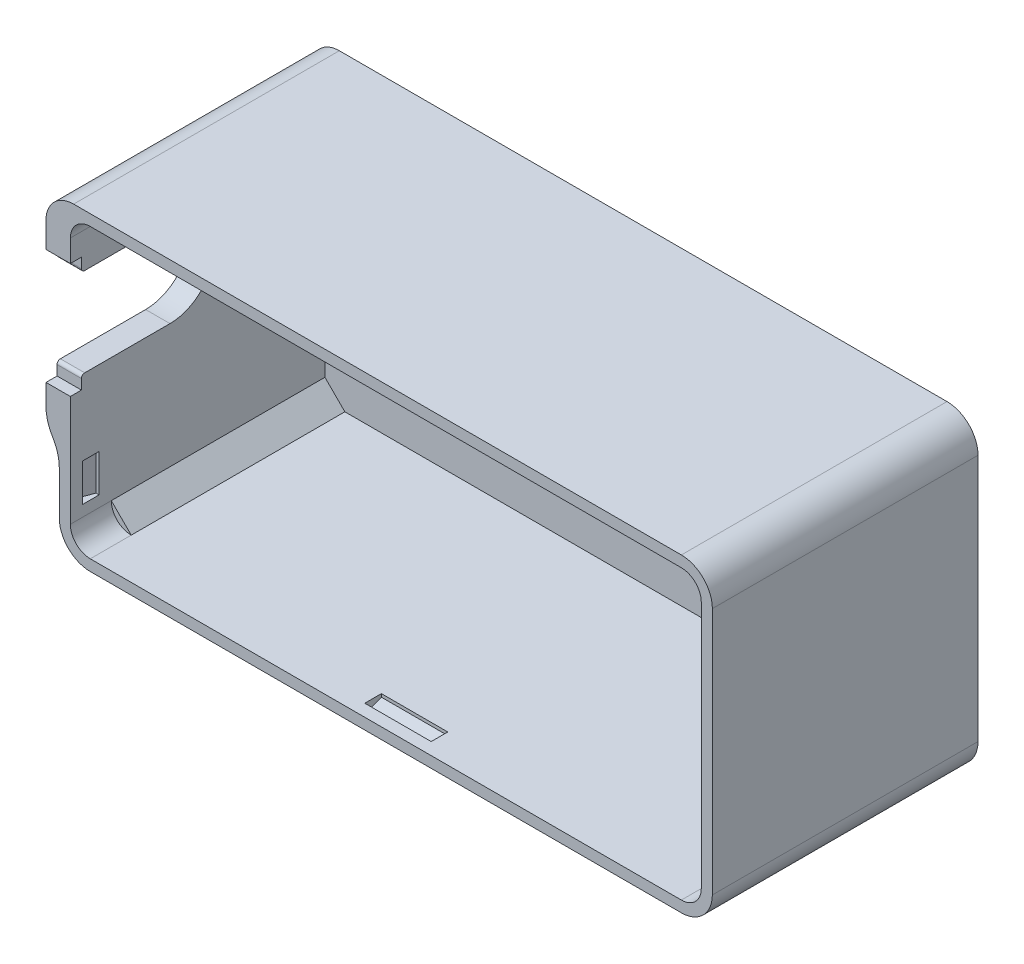
SolidWorks part; units mm, degrees
ref_plane "前视基准面" through (0, 0, 0) normal (0, 0, 1) x (1, 0, 0)
ref_plane "上视基准面" through (0, 0, 0) normal (0, 1, 0) x (1, 0, 0)
ref_plane "右视基准面" through (0, 0, 0) normal (1, 0, 0) x (0, 0, -1)
other "Configuration Table"
sketch "草图1" plane through (0, 0, 0) normal (0, 0, 1) x (1, 0, 0)
  line L0 (-26.7, 14) -> (26.7, 14)
  line L1 (-26.7, 13) -> (26.7, 13)
  line L2 (-28.5, 11.2) -> (-28.5, -11.2)
  line L3 (-26.7, -13) -> (26.7, -13)
  line L4 (28.5, 11.2) -> (28.5, -11.2)
  line L5 (-28.5, 13) -> (28.5, -13) construction
  line L6 (-28.5, -13) -> (28.5, 13) construction
  line L7 (29.5, 11.2) -> (29.5, -11.2)
  line L8 (-26.7, -14) -> (26.7, -14)
  line L9 (-29.5, 11.2) -> (-29.5, -11.2)
  arc A0 (26.7, 13) -> (28.5, 11.2) centre (26.7, 11.2) cw
  arc A1 (-28.5, -11.2) -> (-26.7, -13) centre (-26.7, -11.2) ccw
  arc A2 (-26.7, 13) -> (-28.5, 11.2) centre (-26.7, 11.2) ccw
  arc A3 (26.7, -13) -> (28.5, -11.2) centre (26.7, -11.2) ccw
  arc A4 (26.7, 14) -> (29.5, 11.2) centre (26.7, 11.2) cw
  arc A5 (26.7, -14) -> (29.5, -11.2) centre (26.7, -11.2) ccw
  arc A6 (-29.5, -11.2) -> (-26.7, -14) centre (-26.7, -11.2) ccw
  arc A7 (-26.7, 14) -> (-29.5, 11.2) centre (-26.7, 11.2) ccw
  point P0 (0, 0)
  dimension "D3" = 1.8
  dimension "D1" = 57
  dimension "D2" = 26
  dimension "D4" = 1
extrude "凸台-拉伸1" add sketch "草图1" along normal blind 23
sketch "草图2" plane through (0, 0, 0) normal (0, 0, -1) x (-1, 0, 0)
  line L4 (26.7, 14) -> (-26.7, 14)
  line L5 (-29.5, 11.2) -> (-29.5, -11.2)
  line L6 (-26.7, -14) -> (26.7, -14)
  line L7 (29.5, -11.2) -> (29.5, 11.2)
  line L8 (26.7, 14) -> (-26.7, 14)
  line L9 (-29.5, 11.2) -> (-29.5, -11.2)
  line L10 (-26.7, -14) -> (26.7, -14)
  line L11 (29.5, -11.2) -> (29.5, 11.2)
  arc A4 (29.5, 11.2) -> (26.7, 14) centre (26.7, 11.2) ccw
  arc A5 (-26.7, 14) -> (-29.5, 11.2) centre (-26.7, 11.2) ccw
  arc A6 (-29.5, -11.2) -> (-26.7, -14) centre (-26.7, -11.2) ccw
  arc A7 (26.7, -14) -> (29.5, -11.2) centre (26.7, -11.2) ccw
  arc A8 (29.5, 11.2) -> (26.7, 14) centre (26.7, 11.2) ccw
  arc A9 (-26.7, 14) -> (-29.5, 11.2) centre (-26.7, 11.2) ccw
  arc A10 (-29.5, -11.2) -> (-26.7, -14) centre (-26.7, -11.2) ccw
  arc A11 (26.7, -14) -> (29.5, -11.2) centre (26.7, -11.2) ccw
  dimension "D1" = 0
extrude "凸台-拉伸2" add sketch "草图2" along normal blind 1
sketch "草图3" plane through (-29.5, 0, 0) normal (-1, 0, 0) x (0, 0, 1)
  line L0 (0, 0) -> (35.2795, 0) construction
  line L1 (23, 11.2) -> (23, -11.2) construction
  line L2 (14, 8) -> (25.2408, 8)
  line L3 (14, 0) -> (25.2408, 0)
  line L4 (25.2408, 0) -> (25.2408, 8)
  arc A0 (14, 8) -> (14, 0) centre (14, 4) ccw
  circle A1 centre (14, 4) radius 7 construction
  dimension "D1" = 8
  dimension "D4" = 14
  dimension "D2" = 9
  dimension "D3" = 4
extrude "切除-拉伸1" cut sketch "草图3" against normal blind 20
sketch "草图5" plane through (-29.5, 0, 0) normal (-1, 0, 0) x (0, 0, 1)
  line L0 (23, 11.2) -> (23, 8) construction
  line L1 (22, 9.2) -> (25.765, 9.2)
  line L2 (22, 9.2) -> (22, -1.2)
  line L3 (22, -1.2) -> (25.765, -1.2)
  line L4 (25.765, 9.2) -> (25.765, -1.2)
  line L5 (22, 9.2) -> (25.765, -1.2) construction
  line L6 (22, -1.2) -> (25.765, 9.2) construction
  line L7 (23, 8) -> (14, 8) construction
  line L8 (14, 0) -> (23, 0) construction
  point P0 (23.8825, 4)
  dimension "D1" = 1
  dimension "D2" = 1.2
  dimension "D3" = 1.2
extrude "切除-拉伸3" cut sketch "草图5" against normal blind 10
sketch "草图6" plane through (0, 0, 0) normal (0, 1, 0) x (1, 0, 0)
  line L0 (-28.5, -21.9) -> (-29.2, -21.9)
  line L1 (-28.5, -22) -> (-28.5, -14) construction
  line L2 (-29.2, -21.55) -> (-28.7814, -20.4)
  line L3 (-28.7814, -20.4) -> (-28.5, -20.4)
  line L4 (-29.5, -23) -> (-28.5, -23) construction
  line L5 (-28.5, -20.4) -> (-28.5, -21.9)
  line L8 (-29.2, -21.55) -> (-29.2, -21.9)
  dimension "D5" = 1.5
  dimension "D1" = 20
  dimension "D2" = 0.35
  dimension "D3" = 1.1
  dimension "D4" = 0.7
extrude "切除-拉伸4" cut sketch "草图6" along normal blind 3.4 from offset 6.8
mirror "镜向1" about plane through (0, 0, 0) normal (0, 1, 0) of "切除-拉伸4"
mirror "镜向2" about plane through (0, 0, 0) normal (1, 0, 0) of "切除-拉伸4", "镜向1"
fillet "圆角2" radius 0.3 2 edges at (-29, 0, 22) (-29, 8, 22)
sketch "草图9" plane through (0, 0, 0) normal (0, 0, 1) x (1, 0, 0)
  line L2 (-28.5, 11.2) -> (-26.7, 13)
  line L3 (0, 0) -> (8.5039, 0) construction
  line L4 (0, 0) -> (0, -3.4058) construction
  line L5 (0, -3.4058) -> (8.5039, -3.4058) construction
  line L6 (8.5039, 0) -> (8.5039, -3.4058) construction
  line L9 (28.5, 11.2) -> (26.7, 13)
  line L13 (28.5, -11.2) -> (26.7, -13)
  line L14 (-28.5, -11.2) -> (-26.7, -13)
  arc A9 (-26.7, 13) -> (-28.5, 11.2) centre (-26.7, 11.2) ccw construction
  arc A10 (-26.7, 13) -> (-28.5, 11.2) centre (-26.7, 11.2) ccw
  arc A11 (26.7, 13) -> (28.5, 11.2) centre (26.7, 11.2) cw
  arc A12 (26.7, -13) -> (28.5, -11.2) centre (26.7, -11.2) ccw
  arc A13 (-26.7, -13) -> (-28.5, -11.2) centre (-26.7, -11.2) cw
extrude "凸台-拉伸3" add sketch "草图9" along normal blind 19.3
sketch "草图11" plane through (0, 0, 23) normal (0, 0, 1) x (1, 0, 0)
  line L0 (-30.7, -3.0681) -> (-30.7, 11.5)
  line L1 (26.7, 14) -> (-26.7, 14) construction
  line L2 (-28.5, 11.2) -> (-28.5, -11.2) construction
  line L3 (-30.1499, -5.0924) -> (-30.0501, -5.2625)
  line L4 (-29.5, -1.2) -> (-29.5, -11.2) construction
  line L5 (-29.5, -7.2869) -> (-29.5, -11.2) construction
  line L6 (-26.7, 14) -> (-28.2, 14)
  line L7 (-29.5, 11.2) -> (-29.5, -7.2869)
  arc A0 (-28.2, 14) -> (-30.7, 11.5) centre (-28.2, 11.5) ccw
  arc A1 (-30.0501, -5.2625) -> (-29.5, -7.2869) centre (-33.5, -7.2869) cw
  arc A2 (-30.7, -3.0681) -> (-30.1499, -5.0924) centre (-26.7, -3.0681) ccw
  arc A3 (-26.7, 14) -> (-29.5, 11.2) centre (-26.7, 11.2) ccw construction
  arc A4 (-26.7, 14) -> (-29.5, 11.2) centre (-26.7, 11.2) ccw
  point P16 (-29.5, -6.2)
  dimension "D2" = 4
  dimension "D3" = 4
  dimension "D4" = 5
  dimension "D1" = 2.2
extrude "凸台-拉伸4" add sketch "草图11" against normal up to vertex (24 mm away)
sketch "草图12" plane through (-29.5, 0, 0) normal (1, 0, 0) x (0, 0, -1)
  line L0 (-22, 8.3) -> (-22, 9.2) construction
  line L1 (-22, 9.2) -> (-23, 9.2) construction
  line L2 (-14, 8) -> (-20.4, 8) construction
  line L3 (-21.7, 0) -> (-14, 0) construction
  line L4 (-22, -1.2) -> (-22, -0.3) construction
  line L5 (-23, -1.2) -> (-22, -1.2) construction
  line L6 (-22, 8.3) -> (-22, 9.2)
  line L7 (-22, 9.2) -> (-23, 9.2)
  line L8 (-14, 8) -> (-20.4, 8)
  line L9 (-21.7, 0) -> (-14, 0)
  line L10 (-22, -1.2) -> (-22, -0.3)
  line L11 (-23, -1.2) -> (-22, -1.2)
  line L12 (-21.7, 8) -> (-14, 8) construction
  line L13 (-21.7, 8) -> (-14, 8)
  line L14 (-21.7, 8) -> (-20.4, 8)
  line L15 (-23, 9.2) -> (-23, -1.2)
  arc A0 (-14, 0) -> (-14, 8) centre (-14, 4) ccw construction
  arc A1 (-21.7, 0) -> (-22, -0.3) centre (-21.7, -0.3) ccw construction
  arc A2 (-14, 0) -> (-14, 8) centre (-14, 4) ccw
  arc A3 (-21.7, 0) -> (-22, -0.3) centre (-21.7, -0.3) ccw
  arc A4 (-22, 8.3) -> (-21.7, 8) centre (-21.7, 8.3) ccw construction
  arc A5 (-22, 8.3) -> (-21.7, 8) centre (-21.7, 8.3) ccw
  line M2 (-23, -1.2) -> (-22, -1.2)
  line M3 (-22, -1.2) -> (-22, -0.3)
  arc M4 (-22, -0.3) -> (-21.7, 0) centre (-21.7, -0.3) cw
  line M5 (-21.7, 0) -> (-14, 0)
  arc M6 (-14, 0) -> (-14, 8) centre (-14, 4) ccw
  line M7 (-14, 8) -> (-21.7, 8)
  arc M8 (-21.7, 8) -> (-22, 8.3) centre (-21.7, 8.3) cw
  line M9 (-22, 8.3) -> (-22, 9.2)
  line M10 (-22, 9.2) -> (-23, 9.2)
  line M11 (-23, 9.2) -> (-23, -1.2)
extrude "切除-拉伸5" cut sketch "草图12" against normal blind 10 contours M11 M2 M3 M4 M5 M6 M7 M8 M9 M10
other "删除面1" face at (-28.9907, 9.1, 20.975)
sketch "草图13" plane through (0, 8, 0) normal (0, -1, 0) x (1, 0, 0)
  line L5 (-28.5, 20.4) -> (-28.5, 21.9)
  line L6 (-28.5, 21.9) -> (-29.2, 21.9)
  line L7 (-29.2, 21.9) -> (-29.2, 21.55)
  line L8 (-29.2, 21.55) -> (-28.7814, 20.4)
  line L9 (-28.7814, 20.4) -> (-28.5, 20.4)
  line L10 (-28.5, 20.4) -> (-28.5, 21.9)
  line L11 (-28.5, 21.9) -> (-29.2, 21.9)
  line L12 (-29.2, 21.9) -> (-29.2, 21.55)
  line L13 (-29.2, 21.55) -> (-28.7814, 20.4)
  line L14 (-28.7814, 20.4) -> (-28.5, 20.4)
  dimension "D1" = 0
extrude "凸台-拉伸5" add sketch "草图13" against normal up to vertex
sketch "草图14" plane through (-29.2, 0, 0) normal (-1, 0, 0) x (0, 0, 1)
  line L0 (21.7, 8) -> (22.1142, 8)
  line L1 (22.1142, 8) -> (22, 8.3)
  arc A0 (21.7, 8) -> (22, 8.3) centre (21.7, 8.3) ccw construction
  arc A1 (21.7, 8) -> (22, 8.3) centre (21.7, 8.3) ccw
extrude "切除-拉伸6" cut sketch "草图14" against normal blind 5
sketch "草图10" plane through (0, 0, 0) normal (-1, 0, 0) x (0, 0, 1)
  line L0 (21.9, -13.7) -> (21.9, -13)
  line L1 (19.3, -13) -> (0, -13) construction
  line L2 (21.55, -12.3) -> (20.4, -12.7186) construction
  line L3 (20.4, -13) -> (20.4, -13.2814)
  line L4 (23, -14) -> (23, -11.2) construction
  line L5 (20.4, -13) -> (21.9, -13)
  line L8 (21.55, -12.3) -> (21.9, -12.3) construction
  line L9 (21.55, -13.7) -> (21.9, -13.7)
  line L10 (21.55, -13.7) -> (20.4, -13.2814)
  point P3 (7.8972, -12.3)
  point P4 (7.1697, -12.5914)
  dimension "D5" = 20
  dimension "D1" = 1.5
  dimension "D2" = 0.7
  dimension "D3" = 0.35
  dimension "D4" = 1.1
extrude "切除-拉伸7" cut sketch "草图10" against normal mid plane 6
mirror "镜向3" about plane through (0, 0, 0) normal (0, 1, 0) of "切除-拉伸7"
